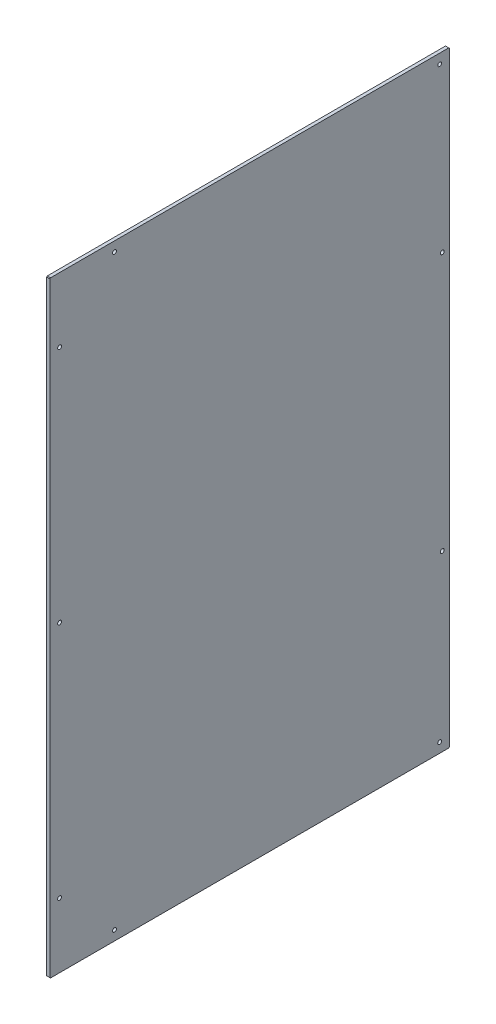
SolidWorks part; units mm, degrees
material "PC(透明)"
ref_plane "前基準面" through (0, 0, 0) normal (0, 0, 1) x (1, 0, 0)
ref_plane "上基準面" through (0, 0, 0) normal (0, 1, 0) x (1, 0, 0)
ref_plane "右基準面" through (0, 0, 0) normal (1, 0, 0) x (0, 0, -1)
sketch "草图1" plane through (0, 0, 0) normal (1, 0, 0) x (0, 0, -1)
  line L1 (309, 469) -> (-309, 469)
  line L2 (309, 469) -> (309, -469)
  line L3 (309, -469) -> (-309, -469)
  line L4 (-309, 469) -> (-309, -469)
  line L5 (309, 469) -> (-309, -469) construction
  line L6 (309, -469) -> (-309, 469) construction
  point P0 (0, 0)
  dimension "D1" = 618
  dimension "D2" = 938
extrude "凸台-拉伸1" add sketch "草图1" along normal blind 5
chamfer "倒角1" distance 1 angle 45 4 edges at (2.5, -469, -309) (2.5, -469, 309) (2.5, 469, -309) (2.5, 469, 309)
sketch "草图2" plane through (0, 0, 0) normal (-1, 0, 0) x (0, 0, 1)
  line L0 (-298, 200) -> (-298, -200) construction
  line L1 (-308, 469) -> (308, 469) construction
  line L2 (58.8862, 0) -> (0, 0) construction
  line L3 (0, 0) -> (0, 69.8386) construction
  line L4 (309, 468) -> (309, -468) construction
  line L5 (294, -454) -> (-294, -454) construction
  line L6 (294, -454) -> (294, 454) construction
  line L7 (294, 454) -> (-294, 454) construction
  line L8 (-294, -454) -> (-294, 454) construction
  line L9 (294, -454) -> (-294, 454) construction
  line L10 (294, 454) -> (-294, -454) construction
  line L11 (-308, 469) -> (308, 469) construction
  line L12 (308, -469) -> (-308, -469) construction
  line L13 (-309, -468) -> (-309, 468) construction
  line L14 (-298, 0) -> (-309, 0) construction
  circle A0 centre (-294, 454) radius 3
  circle A1 centre (-294, -454) radius 3
  circle A2 centre (294, -454) radius 3 construction
  circle A3 centre (294, 454) radius 3 construction
  circle A4 centre (209, 454) radius 3
  circle A5 centre (294, 369) radius 3
  circle A6 centre (294, -369) radius 3
  circle A7 centre (209, -454) radius 3
  circle A8 centre (294, 0) radius 3
  circle A9 centre (-294, 0) radius 3 construction
  circle A10 centre (-298, 200) radius 3
  circle A11 centre (-298, -200) radius 3
  dimension "D1" = 6
  dimension "D4" = 100
  dimension "D5" = 100
  dimension "D2" = 15
  dimension "D3" = 15
  dimension "D6" = 100
  dimension "D7" = 15
  dimension "D8" = 11
  dimension "D9" = 400
extrude "切除-拉伸1" cut sketch "草图2" against normal through all
